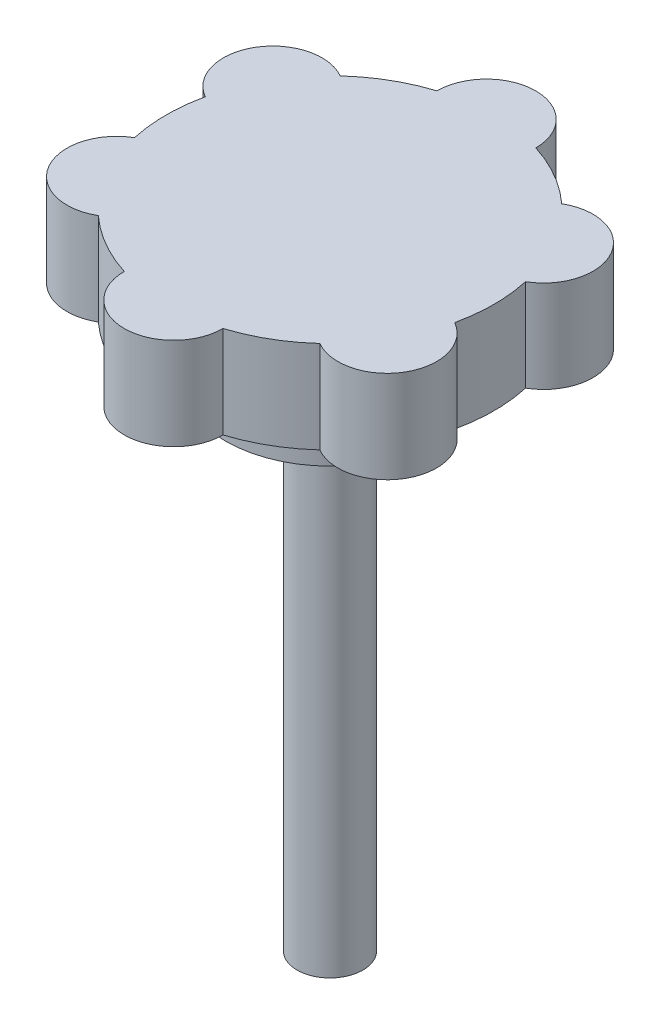
from build123d import *

# Parameters (mm, degrees)
BOSS_EXTRUDE1_DEPTH = 5.6
SKETCH2_R           = 6.35
BOSS_EXTRUDE2_DEPTH = 3.4
SKETCH3_R           = 2
BOSS_EXTRUDE3_DEPTH = 30


with BuildPart() as part:
    # Sketch1 → Boss-Extrude1 (new body)
    with BuildSketch(Plane(origin=(0, 0, 0), x_dir=(1, 0, 0), z_dir=(0, 1, 0))):
        with BuildLine():
            Line((-9.72424134, -2.15192377), (-9.725740285, -2.152789186))
            ThreePointArc((-9.725740285, -2.152789186), (-10.823817926, -6.250865027), (-6.725742085, -7.348942669))
            Line((-6.725742085, -7.348942669), (-6.723420775, -7.34760246))
            ThreePointArc((-6.723420775, -7.34760246), (-4.978167749, -8.626268935), (-2.998, -9.497952231))
            Line((-2.998, -9.497952231), (-2.998, -9.5))
            ThreePointArc((-2.998, -9.5), (0.002000003, -12.499999996), (3.002, -9.499999993))
            Line((3.002, -9.499999993), (3.002, -9.497636397))
            ThreePointArc((3.002, -9.497636397), (4.982303032, -8.625613539), (6.727581168, -7.346540363))
            Line((6.727581168, -7.346540363), (6.728741336, -7.347210186))
            ThreePointArc((6.728741336, -7.347210186), (10.826817547, -6.249133975), (9.728741336, -2.151057763))
            Line((9.728741336, -2.151057763), (9.727581168, -2.15038794))
            ThreePointArc((9.727581168, -2.15038794), (9.962651964, 0.001128196), (9.727467916, 2.152631955))
            ThreePointArc((9.727467916, 2.152631955), (10.825817547, 6.250866025), (6.727194396, 7.348626461))
            ThreePointArc((6.727194396, 7.348626461), (4.981167779, 8.628000969), (3, 9.5))
            ThreePointArc((3, 9.5), (2e-09, 12.5), (-3, 9.499052498))
            ThreePointArc((-3, 9.499052498), (-4.980665222, 8.626558938), (-6.726128008, 7.346856081))
            ThreePointArc((-6.726128008, 7.346856081), (-10.824817547, 6.249133975), (-9.726741336, 2.151057764))
            Line((-9.726741336, 2.151057764), (-9.725033927, 2.150071991))
            ThreePointArc((-9.725033927, 2.150071991), (-9.959651798, -0.000969188), (-9.72424134, -2.15192377))
        make_face()
    extrude(amount=BOSS_EXTRUDE1_DEPTH)

    # Sketch2 → Boss-Extrude2 (add)
    with BuildSketch(Plane.XZ):
        with Locations(Location((0, 0, 0), (0, 0, 90))):
            Circle(SKETCH2_R)
    extrude(amount=BOSS_EXTRUDE2_DEPTH)

    # Sketch3 → Boss-Extrude3 (add)
    with BuildSketch(Plane.XZ.offset(3.4)):
        with Locations(Location((0, 0, 0), (0, 0, 270))):
            Circle(SKETCH3_R)
    extrude(amount=BOSS_EXTRUDE3_DEPTH)


solid = part.part
